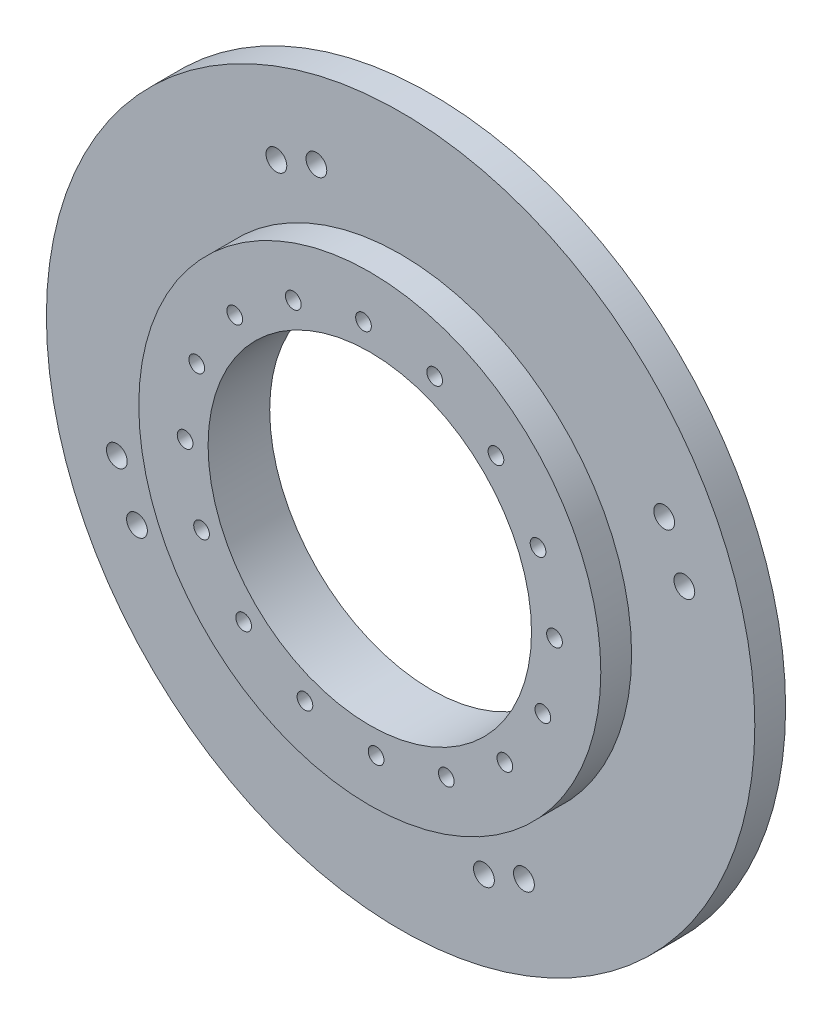
from build123d import *

# Parameters (mm, degrees)
SKETCH_1_R               = 230
EXTRUDE_1_DEPTH          = 10
SKETCH_2_R               = 105
CUT_EXTRUDE_1_DEPTH      = 326.883414736
SKETCH_3_R               = 150
SKETCH_3_R_2             = 105
EXTRUDE_2_DEPTH          = 20
HOLE_WIZARD_M12_1_D      = 10.2
PATTERN_CIRCULAR_1_COUNT = 16
HOLE_WIZARD_M12_1_2_D    = 13.5


with BuildPart() as part:
    # 草图1 → 凸台-拉伸1 (new, symmetric)
    with BuildSketch(Plane.XY):
        Circle(SKETCH_1_R)
    extrude(amount=EXTRUDE_1_DEPTH, both=True)

    # 草图2 → 切除-拉伸1 (cut, through all)
    with BuildSketch(Plane(origin=(0, 0, -10), x_dir=(-1, 0, 0), z_dir=(0, 0, -1))):
        Circle(SKETCH_2_R)
    extrude(amount=-CUT_EXTRUDE_1_DEPTH, mode=Mode.SUBTRACT)

    # 草图3 → 凸台-拉伸2 (add)
    with BuildSketch(Plane.XY.offset(10)):
        Circle(SKETCH_3_R)
        with Locations(Location((0, 0, 0), (0, 0, 180))):
            Circle(SKETCH_3_R_2, mode=Mode.SUBTRACT)
    extrude(amount=EXTRUDE_2_DEPTH)

    # Hole Wizard M12 _1 (through all)
    with Locations(Plane.XY.offset(30)):
        with Locations((112.365701655, -42.118275031)):
            hole_wizard_m12_1 = Hole(HOLE_WIZARD_M12_1_D / 2)

    # 阵列(圆周)1: Hole Wizard M12 _1 ×16 about axis
    pattern_circular_1_axis = Axis((0, 0, 0), (0, 0, 1))
    for i in range(1, PATTERN_CIRCULAR_1_COUNT):
        add(hole_wizard_m12_1.rotate(pattern_circular_1_axis, i * 360 / PATTERN_CIRCULAR_1_COUNT), mode=Mode.SUBTRACT)

    # Hole Wizard M12 _1 2 (through all)
    with Locations(Plane.XY.offset(10)):
        with Locations((54.118704372, -171.719208219), (80.088559574, -161.251800671), (171.165878787, 87.858133743), (184.250138222, 55.395814741), (-171.165880115, -87.858134279), (-184.25013955, -55.395815276), (-80.649167813, 162.642677508), (-54.679312611, 173.110085056)):
            Hole(HOLE_WIZARD_M12_1_2_D / 2)


solid = part.part
